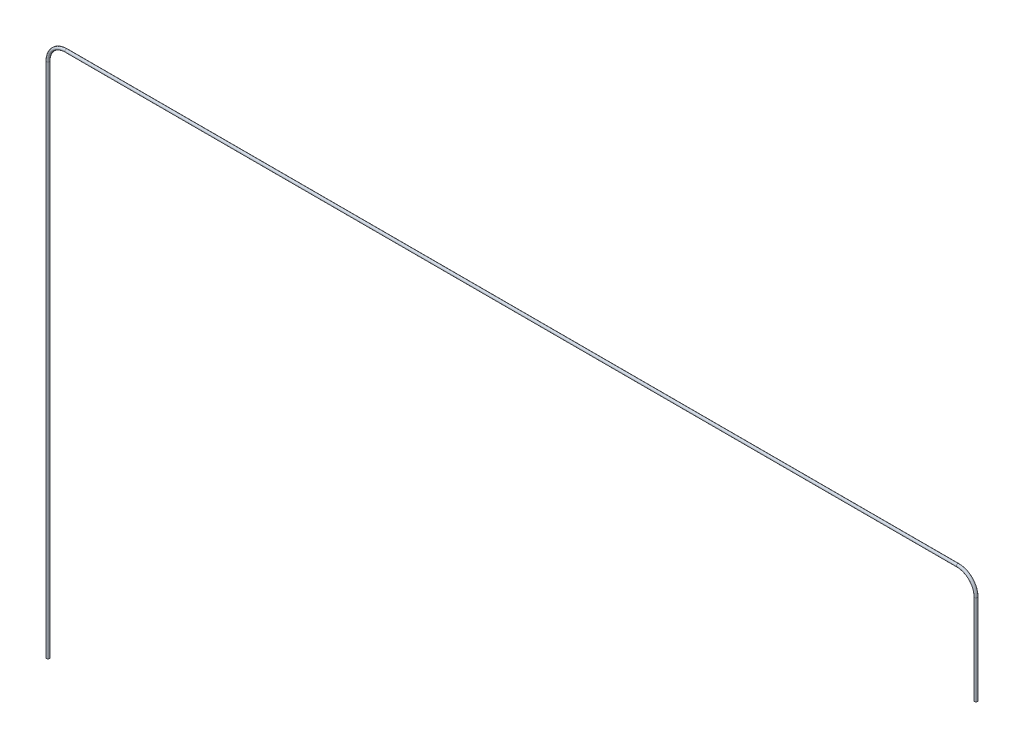
from build123d import *

# Parameters (mm, degrees)
SKETCH2_R = 3.25


with BuildPart() as part:
    # Sweep1: sweep along a path in Sketch1
    with BuildLine(Plane.XY) as sweep1_path:
        Line((0, 0), (0, 1193))
        ThreePointArc((0, 1193), (12.30151519, 1222.69848481), (42, 1235))
        Line((42, 1235), (2100, 1235))
        ThreePointArc((2100, 1235), (2129.69848481, 1222.69848481), (2142, 1193))
        Line((2142, 1193), (2142, 985))
    # Sketch2 → Sweep1 (sweep)
    with BuildSketch(Plane(origin=(0, 0, 0), x_dir=(1, 0, 0), z_dir=(0, 1, 0))):
        Circle(SKETCH2_R)
    sweep(path=sweep1_path.line)


solid = part.part
